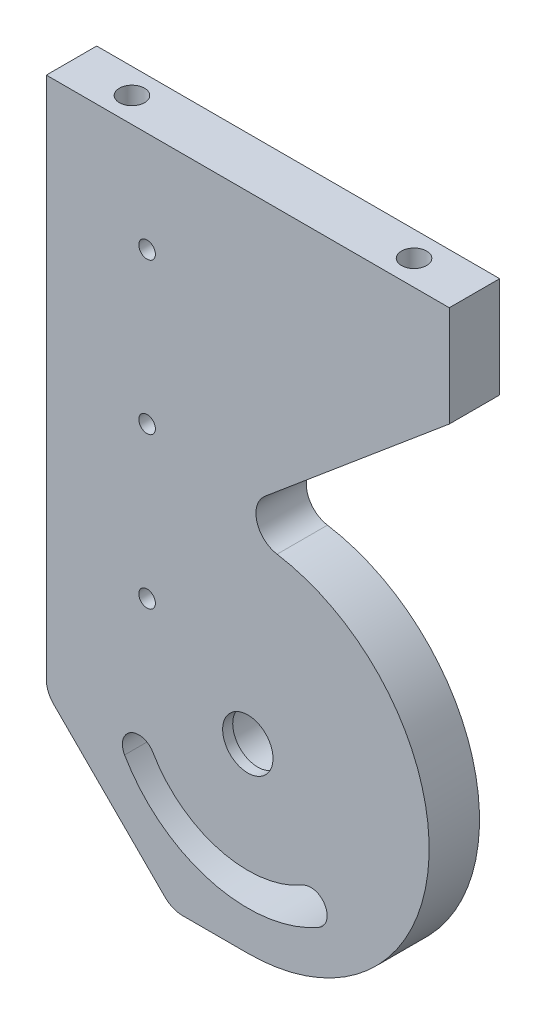
SolidWorks part; units mm, degrees
material "6061"
ref_plane "前视基准面" through (0, 0, 0) normal (0, 0, 1) x (1, 0, 0)
ref_plane "上视基准面" through (0, 0, 0) normal (0, 1, 0) x (1, 0, 0)
ref_plane "右视基准面" through (0, 0, 0) normal (1, 0, 0) x (0, 0, -1)
sketch "草图1" plane through (0, 0, 0) normal (0, 0, 1) x (1, 0, 0)
  line L1 (-40, -85) -> (40, -85)
  line L2 (-40, -85) -> (-40, 85)
  line L3 (-40, 85) -> (40, 85)
  line L4 (40, -85) -> (40, 85)
  line L5 (-40, -85) -> (40, 85) construction
  line L6 (-40, 85) -> (40, -85) construction
  point P0 (0, 0)
  dimension "D1" = 80
  dimension "D2" = 170
extrude "凸台-拉伸1" add sketch "草图1" along normal mid plane 10
hole_wizard "孔1" positions "草图5" profile "草图4" legacy end condition through all
sketch "草图5" plane through (0, 0, -5) normal (0, 0, -1) x (-1, 0, 0)
  point P0 (0, -10)
  dimension "D1" = 10
sketch "草图4" plane through (0, -10, -5) normal (1, 0, 0) x (0, 1, 0)
  line L0 (0, 0) -> (0, 10)
  line L1 (0, 10) -> (5, 10)
  line L2 (5, 10) -> (5, 8)
  line L3 (5, 8) -> (6, 8)
  line L4 (6, 8) -> (6, 0)
  line L5 (6, 0) -> (0, 0)
  line L6 (0, 110) -> (0, -10) construction
  dimension "直径" = 10
  dimension "深度" = 10
  dimension "柱坑直径" = 12
  dimension "柱坑深度" = 8
sketch "草图6" plane through (0, 0, -5) normal (0, 0, -1) x (-1, 0, 0)
  line L0 (0, -10) -> (-12.5, -31.6506) construction
  line L1 (0, -10) -> (21.6506, -22.5) construction
  line L2 (0, -10) -> (0, -48.1062) construction
  circle A0 centre (0, -10) radius 25 construction
  arc A1 (-14.125, -34.4652) -> (24.4652, -24.125) centre (0, -10) ccw
  arc A2 (-10.875, -28.8361) -> (18.8361, -20.875) centre (0, -10) ccw
  arc A3 (-10.875, -28.8361) -> (-14.125, -34.4652) centre (-12.5, -31.6506) ccw
  arc A4 (24.4652, -24.125) -> (18.8361, -20.875) centre (21.6506, -22.5) ccw
  circle A5 centre (0, -10) radius 21.75 construction
  circle A6 centre (0, -10) radius 28.25 construction
  dimension "D1" = 50
  dimension "D2" = 30
  dimension "D3" = 60
  dimension "D4" = 3.25
extrude "切除-拉伸2" cut sketch "草图6" against normal through all
sketch "草图11" plane through (0, 0, -5) normal (0, 0, -1) x (-1, 0, 0)
  line L0 (0, -46) -> (15, -46)
  line L2 (15, -46) -> (40, -21)
  line L3 (40, -85) -> (-40, -85) construction
  line L4 (7.3928, 25.2328) -> (-40, 65)
  line L5 (-40, -85) -> (-40, 85) construction
  line L6 (-40, 65) -> (-40, -85)
  line L7 (-40, -85) -> (40, -85)
  line L8 (40, -85) -> (40, -21)
  line L9 (40, 85) -> (40, -85) construction
  line L10 (-40, 85) -> (40, 85) construction
  arc A0 (7.3928, 25.2328) -> (0, -46) centre (0, -10) ccw
  dimension "D1" = 72
  dimension "D2" = 130
  dimension "D3" = 25
  dimension "D4" = 45
  dimension "D5" = 20
extrude "切除-拉伸4" cut sketch "草图11" against normal through all
fillet "圆角1" radius 5 3 edges at (-7.3928, 25.2328, 0) (-40, -21, 0) (-15, -46, 0)
hole_wizard "M6 螺纹孔1" positions "草图15" profile "草图14" tap size "M6" standard "GB"
sketch "草图15" plane through (0, 85, 0) normal (0, 1, 0) x (1, 0, 0)
  point P0 (-28, 0)
  point P2 (28, 0)
  dimension "D1" = 56
  dimension "D2" = 28
sketch "草图14" plane through (-28, 85, 0) normal (1, 0, 0) x (0, 0, 1)
  line L0 (0, 0) -> (0, 18.5022)
  line L1 (0, 18.5022) -> (2.5, 17)
  line L2 (2.5, 17) -> (2.5, 0)
  line L5 (2.5, 0) -> (0, 0)
  line L10 (0, 18.5022) -> (-2.5, 17) construction
  line L11 (0, -6.35) -> (0, 107.95) construction
  dimension "螺纹孔钻头直径" = 5
  dimension "螺纹孔钻头深度" = 17
  dimension "导头角度" = 118
cosmetic thread "孔螺蚊线1" parameters "D1"=12, "D2"=6
cosmetic thread "孔螺蚊线2" parameters "D1"=12, "D2"=6
hole_wizard "M4 螺纹孔1" positions "草图16" profile "草图17" tap size "M4" standard "GB" end condition through all
sketch "草图16" plane through (0, 0, 5) normal (0, 0, 1) x (1, 0, 0)
  line L0 (-20, 85) -> (-20, -85.9057) construction
  line L1 (40, 85) -> (-40, 85) construction
  line L3 (-40, 85) -> (-40, -18.9289) construction
  point P0 (-20, 65)
  point P11 (-20, 35)
  point P13 (-20, 5)
  dimension "D1" = 20
  dimension "D2" = 20
  dimension "D3" = 30
  dimension "D4" = 30
sketch "草图17" plane through (-20, 65, 5) normal (1, 0, 0) x (0, -1, 0)
  line L0 (0, 0) -> (0, 10)
  line L1 (0, 10) -> (1.65, 10)
  line L2 (1.65, 10) -> (1.65, 0)
  line L5 (1.65, 0) -> (0, 0)
  line L11 (0, -6.35) -> (0, 107.95) construction
  dimension "通孔螺纹孔钻头直径" = 3.3
  dimension "通孔螺纹孔钻头深度" = 10
cosmetic thread "孔螺蚊线3" parameters "D2"=4
cosmetic thread "孔螺蚊线4" parameters "D2"=4
cosmetic thread "孔螺蚊线5" parameters "D2"=4
